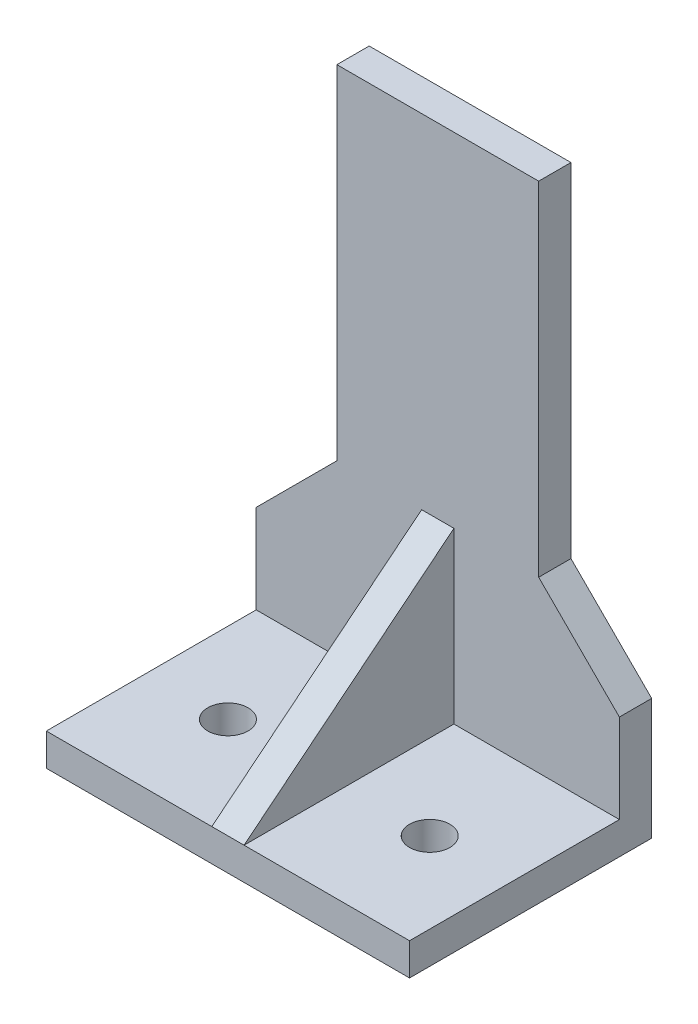
SolidWorks part; units mm, degrees
ref_plane "前视基准面" through (0, 0, 0) normal (0, 0, 1) x (1, 0, 0)
ref_plane "上视基准面" through (0, 0, 0) normal (0, 1, 0) x (1, 0, 0)
ref_plane "右视基准面" through (0, 0, 0) normal (1, 0, 0) x (0, 0, -1)
sketch "草图1" plane through (0, 0, 0) normal (0, 0, 1) x (1, 0, 0)
  line L0 (0, 0) -> (90, 0)
  line L1 (90, 0) -> (90, 30)
  line L2 (0, 0) -> (0, 30)
  line L4 (45, 135) -> (70, 135)
  line L5 (45, 135) -> (20, 135)
  line L6 (20, 135) -> (20, 50)
  line L7 (70, 135) -> (70, 50)
  line L8 (20, 50) -> (0, 30)
  line L9 (70, 50) -> (90, 30)
extrude "凸台-拉伸2" add sketch "草图1" along normal blind 8
sketch "草图2" plane through (0, 0, 8) normal (0, 0, 1) x (1, 0, 0)
  line L0 (0, 0) -> (0, 8)
  line L1 (0, 30) -> (0, 0) construction
  line L2 (0, 8) -> (90, 8)
  line L3 (90, 0) -> (90, 30) construction
  line L4 (90, 8) -> (90, 0)
  line L5 (0, 0) -> (90, 0) construction
  line L6 (90, 0) -> (0, 0)
extrude "凸台-拉伸3" add sketch "草图2" along normal blind 52
sketch "草图3" plane through (0, 0, 8) normal (0, 0, 1) x (1, 0, 0)
  line L0 (45, 135) -> (45, 8)
  line L1 (70, 135) -> (20, 135) construction
  line L2 (90, 8) -> (0, 8) construction
ref_plane "基准面1" through (45, 0, 0) normal (1, 0, 0) x (0, 0, -1)
sketch "草图4" plane through (45, 0, 0) normal (1, 0, 0) x (0, 0, -1)
  line L0 (-8, 8) -> (-8, 50)
  line L1 (-8, 8) -> (-60, 8)
  line L2 (-60, 8) -> (-8, 50)
extrude "凸台-拉伸4" add sketch "草图4" along normal blind 4 and the other way blind 4
sketch "草图5" plane through (0, 8, 0) normal (0, 1, 0) x (1, 0, 0)
  line L0 (0, -60) -> (0, -35)
  line L1 (0, -60) -> (0, -8) construction
  line L2 (0, -35) -> (90, -35)
  line L3 (90, -60) -> (90, -8) construction
  line L5 (90, -35) -> (65, -35)
  line L6 (0, -35) -> (25, -35)
  circle A0 centre (65, -35) radius 5
  circle A1 centre (25, -35) radius 5
extrude "切除-拉伸2" cut sketch "草图5" against normal blind 18 contours L2 A0 | L2 A0 | L6 A1 L2 | L2 A1 L6
sketch "草图6" plane through (0, 8, 0) normal (0, 1, 0) x (1, 0, 0)
  line L0 (25, -35) -> (65, -35)
  line L4 (45, -35) -> (20, -35)
  line L5 (45, -35) -> (70, -35)
  circle A0 centre (20, -35) radius 5
  circle A1 centre (70, -35) radius 5
  circle A2 centre (25, -35) radius 5
  circle A3 centre (65, -35) radius 5
extrude "切除-拉伸3" cut sketch "草图6" against normal blind 10 contours L0 A0
sketch "草图7" plane through (0, 8, 0) normal (0, 1, 0) x (1, 0, 0)
  line L0 (-42.765, -29.1865) -> (140.2667, -34.5041)
  line L2 (72.1214, -16.4418) -> (76.6477, -16.4418)
  line L3 (72.1214, -16.4418) -> (72.1214, -13.9212)
  line L4 (72.1214, -13.9212) -> (76.6477, -13.9212)
  line L5 (76.6477, -16.4418) -> (76.6477, -13.9212)
sketch "草图8" plane through (0, 8, 0) normal (0, 1, 0) x (1, 0, 0)
  line L0 (20, -35) -> (70, -35)
  circle A1 centre (70, -35) radius 5
  circle M1 centre (65, -35) radius 5
extrude "切除-拉伸4" cut sketch "草图8" against normal blind 10 contours A1 M1
sketch "草图9" plane through (0, 8, 0) normal (0, 1, 0) x (1, 0, 0)
  circle A0 centre (20, -35) radius 5
  arc A1 (22.5, -39.3301) -> (22.5, -30.6699) centre (25, -35) ccw
  arc A2 (67.5, -30.6699) -> (67.5, -39.3301) centre (65, -35) ccw
  circle A3 centre (70, -35) radius 5
extrude "凸台-拉伸6" add sketch "草图9" against normal blind 8 contours A0 | A3 A2
